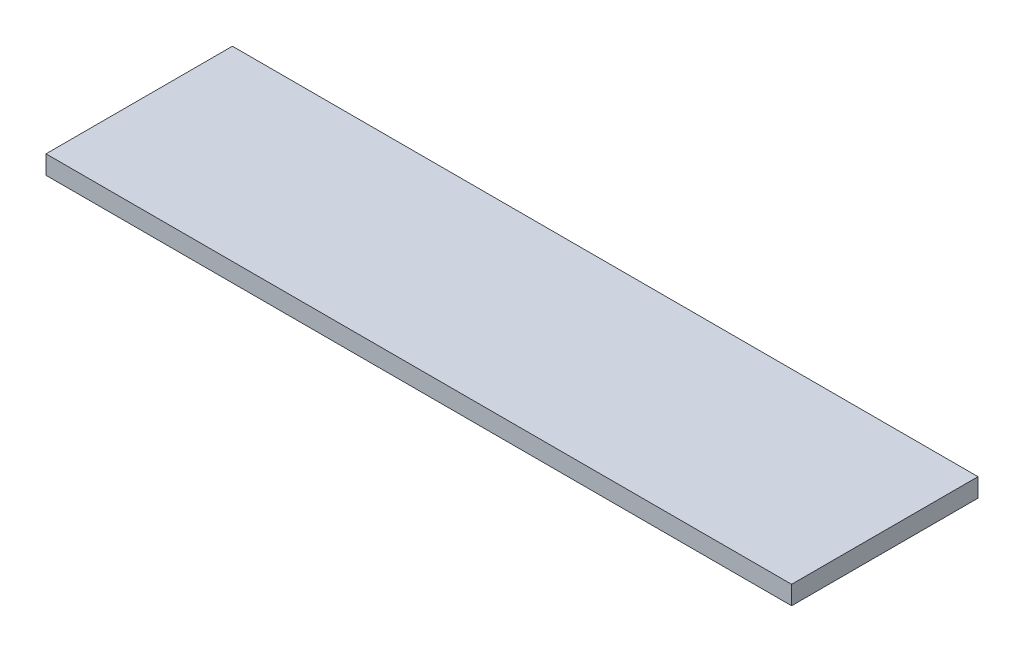
SolidWorks part; units mm, degrees
ref_plane "Front Plane" through (0, 0, 0) normal (0, 0, 1) x (1, 0, 0)
ref_plane "Top Plane" through (0, 0, 0) normal (0, 1, 0) x (1, 0, 0)
ref_plane "Right Plane" through (0, 0, 0) normal (1, 0, 0) x (0, 0, -1)
sketch "Sketch1" plane through (0, 0, 0) normal (0, 1, 0) x (1, 0, 0)
  line L0 (500, 125) -> (-500, -125) construction
  line L1 (-500, 125) -> (500, 125)
  line L2 (-500, 125) -> (-500, -125)
  line L3 (-500, -125) -> (500, -125)
  line L4 (500, 125) -> (500, -125)
  dimension "D1" = 1000
  dimension "D2" = 250
extrude "Extrude1" add sketch "Sketch1" along normal mid plane 25
fillet "Fillet1" [suppressed] radius 30
fillet "Fillet2" [suppressed] radius 2
sketch "Sketch2" [suppressed] plane through (0, 12.5, 0) normal (0, 1, 0) x (1, 0, 0)
  line L2 (498, 125) -> (-498, 125) construction
  line L3 (-240.5, 125) -> (-185.5, 125)
  line L4 (-240.5, 125) -> (-240.5, 70)
  line L5 (-240.5, 70) -> (-185.5, 70)
  line L6 (-185.5, 125) -> (-185.5, 70)
  line L7 (-213, 125) -> (-213, 70) construction
  dimension "D1" = 287
  dimension "D2" = 55
  dimension "D3" = 55
extrude "Cut-Extrude1" [suppressed] cut sketch "Sketch2" against normal through all
pattern_linear "Linear Pattern1" [suppressed] count 2 spacing 400
fillet "Fillet3" [suppressed] radius 10
